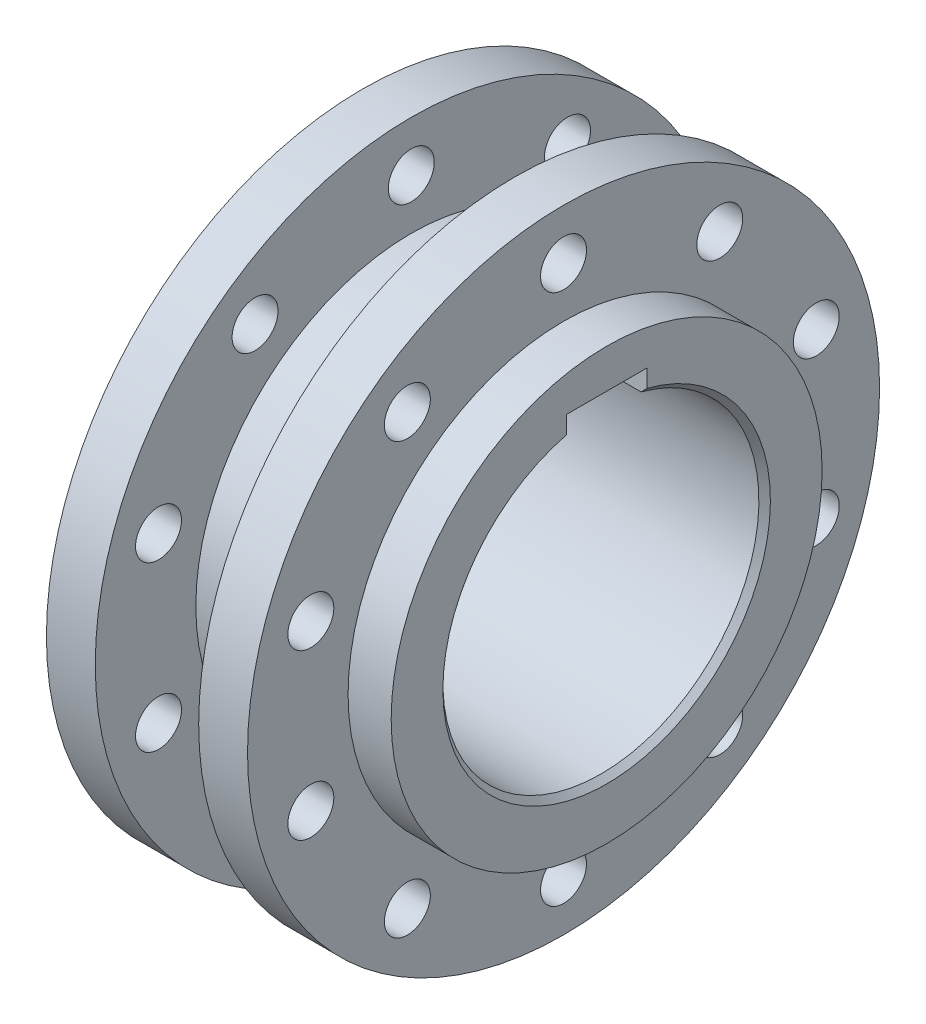
from build123d import *

# Parameters (mm, degrees)
SKETCH2_R          = 8
CUT_EXTRUDE1_DEPTH = 178.270979012
CIRPATTERN1_COUNT  = 10
SKETCH3_W          = 28
SKETCH3_H          = 61.4
CUT_EXTRUDE2_DEPTH = 185.932420089


with BuildPart() as part:
    # Sketch1 → Revolve1 (revolve)
    with BuildSketch(Plane.XY, mode=Mode.PRIVATE) as revolve1_sk:
        Polygon((-50, 57), (-50, 75), (-35, 75), (-35, 110), (-18, 110), (-18, 75), (18, 75), (18, 110), (35, 110), (35, 75), (50, 75), (50, 57), (48, 55), (-48, 55), align=None)
    revolve(revolve1_sk.sketch.rotate(Axis((-54.276945294, 0, 0), (1, 0, 0)), 90), axis=Axis((-54.276945294, 0, 0), (1, 0, 0)))

    # Sketch2 → Cut-Extrude1 (cut, through all)
    with BuildSketch(Plane.ZY.offset(35)):
        with Locations((0, 92.5)):
            Circle(SKETCH2_R)
    cut_extrude1 = extrude(amount=-CUT_EXTRUDE1_DEPTH, mode=Mode.SUBTRACT)

    # CirPattern1: Cut-Extrude1 ×10 about axis
    cirpattern1_axis = Axis((0, 0, 0), (1, 0, 0))
    for i in range(1, CIRPATTERN1_COUNT):
        add(cut_extrude1.rotate(cirpattern1_axis, i * 360 / CIRPATTERN1_COUNT), mode=Mode.SUBTRACT)

    # Sketch3 → Cut-Extrude2 (cut, through all)
    with BuildSketch(Plane(origin=(50, 0, 0), x_dir=(0, 0, -1), z_dir=(1, 0, 0))):
        with Locations((0, 30.7)):
            Rectangle(SKETCH3_W, SKETCH3_H)
    extrude(amount=-CUT_EXTRUDE2_DEPTH, mode=Mode.SUBTRACT)


solid = part.part
